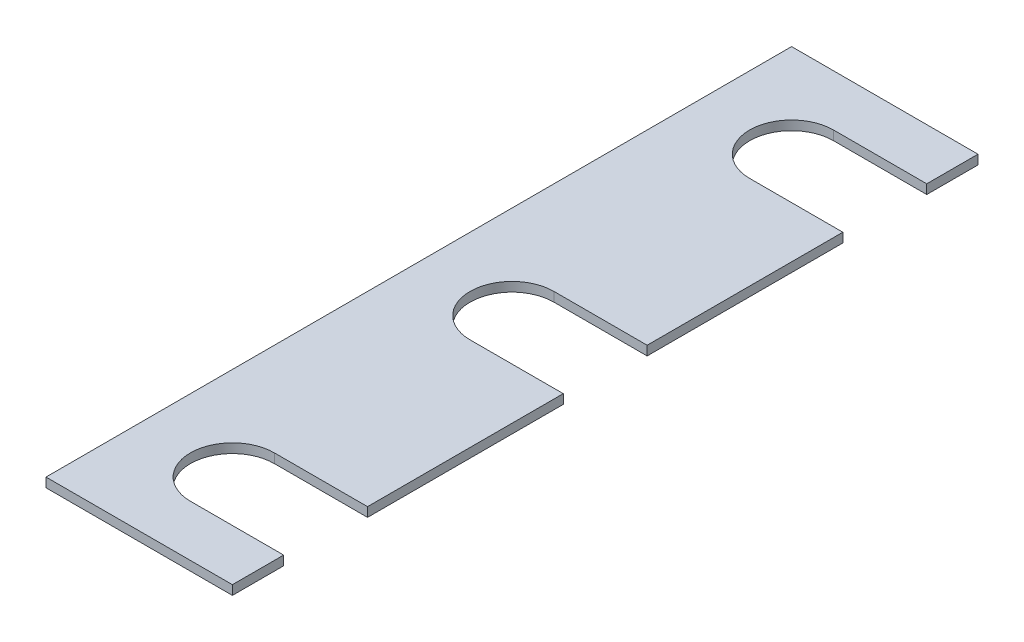
from build123d import *

# Parameters (mm, degrees)
EXTRUDE_1_DEPTH = 2


with BuildPart() as part:
    # 草图1 → 凸台-拉伸1 (new body)
    with BuildSketch(Plane(origin=(0, 0, 0), x_dir=(1, 0, 0), z_dir=(0, 1, 0))):
        with BuildLine():
            Line((0, 9), (20, 9))
            Line((20, 9), (20, 51))
            Line((20, 51), (0, 51))
            ThreePointArc((0, 51), (-9, 60), (0, 69))
            Line((0, 69), (20, 69))
            Line((20, 69), (20, 80))
            Line((20, 80), (-20, 80))
            Line((-20, 80), (-20, -80))
            Line((-20, -80), (20, -80))
            Line((20, -80), (20, -69))
            Line((20, -69), (0, -69))
            ThreePointArc((0, -69), (-9, -60), (0, -51))
            Line((0, -51), (20, -51))
            Line((20, -51), (20, -9))
            Line((20, -9), (0, -9))
            ThreePointArc((0, -9), (-9, 0), (0, 9))
        make_face()
    extrude(amount=EXTRUDE_1_DEPTH)


solid = part.part
